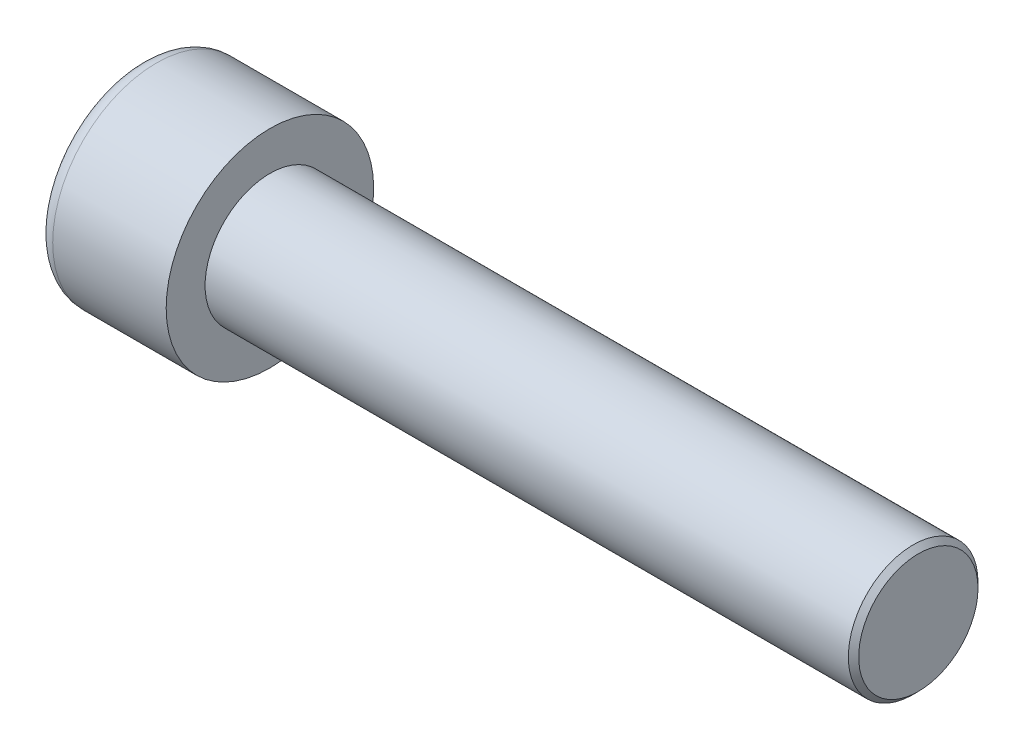
SolidWorks part; units mm, degrees
ref_plane "Front" through (0, 0, 0) normal (0, 0, 1) x (1, 0, 0)
ref_plane "Top" through (0, 0, 0) normal (0, 1, 0) x (1, 0, 0)
ref_plane "Right" through (0, 0, 0) normal (1, 0, 0) x (0, 0, -1)
sketch "Sketch1" plane through (0, 0, 0) normal (1, 0, 0) x (0, 0, -1)
  circle A0 centre (0, 0) radius 8
  dimension "dk" = 16
extrude "BaseHead" add sketch "Sketch1" along normal blind 10
sketch "Sketch2" plane through (10, 0, 0) normal (1, 0, 0) x (0, 0, -1)
  circle A0 centre (0, 0) radius 5
extrude "BaseBody" add sketch "Sketch2" along normal blind 50
cosmetic thread "ThreadCosmetic1" [suppressed] parameters "b"=32, "D2"=8.376
sketch "Sketch3" plane through (0, 0, 0) normal (1, 0, 0) x (0, 0, -1)
  line L1 (4.6188, 0) -> (2.3094, 4)
  line L2 (2.3094, 4) -> (-2.3094, 4)
  line L3 (-2.3094, 4) -> (-4.6188, 0)
  line L4 (-4.6188, 0) -> (-2.3094, -4)
  line L5 (-2.3094, -4) -> (2.3094, -4)
  line L6 (2.3094, -4) -> (4.6188, 0)
  circle A0 centre (0, 0) radius 4 construction
  dimension "s" = 8
  dimension "e" = 9.2376
extrude "HexagonSocket" cut sketch "Sketch3" along normal blind 5
sketch "Sketch4" plane through (-4.1961, 0.75, 0) normal (0, 0, 1) x (-1, 0, 0)
  line L0 (-9.1961, 4.75) -> (-11.5055, 0.75)
  line L2 (-11.5055, 0.75) -> (-9.1961, 0.75)
  line L3 (-9.1961, 0.75) -> (-9.1961, 4.75)
  line L4 (-5.0351, 0.75) -> (0.839, 0.75) construction
  line L5 (-64.1961, 0.75) -> (-14.1961, 0.75) construction
  line L6 (-14.1961, 0.75) -> (-4.1961, 0.75) construction
  dimension "m" = 60
revolve "Cut-Revolve1" cut sketch "Sketch4" angle 360 about L4
fillet "HeadFillet" [suppressed] radius 0.4
fillet "TopFillet" radius 1.25 1 edges at (0, 0, -8)
chamfer "Chamfer1" distance 0.4 angle 45 1 edges at (60, 0, -5)
sketch "Sketch5" plane through (0, 0, 0) normal (0, 0, 1) x (1, 0, 0)
  line L0 (59.6, 4.2968) -> (60.006, 5)
  line L1 (60.006, 5) -> (60.006, 5.812)
  line L2 (60.006, 5.812) -> (59.194, 5.812)
  line L3 (59.194, 5.812) -> (59.194, 5)
  line L4 (59.194, 5) -> (59.6, 4.2968)
  line L5 (0, 0) -> (7.8886, 0) construction
  line L6 (59.6, -5) -> (59.6, 5) construction
revolve "Cut-Revolve10" [suppressed] cut sketch "Sketch5" angle 360 about L5
pattern_linear "LPattern10" [suppressed] count 33 spacing 0.9744 along (1, 0, 0)
equation "\"r1@TopFillet\" = \"d@Sketch2\" / 8"
equation "\"D1@Chamfer1\" = \"r@HeadFillet\""
equation "\"D1@Sketch5\" = \"d@Sketch2\""
equation "\"D2@Sketch5\" =  ( \"d@Sketch2\" - \"D2@ThreadCosmetic1\" )  / 2"
equation "\"D3@LPattern10\" = \"D2@Sketch5\" * 1.2"
equation "\"D1@LPattern10\" = \"b@ThreadCosmetic1\" / \"D3@LPattern10\""
